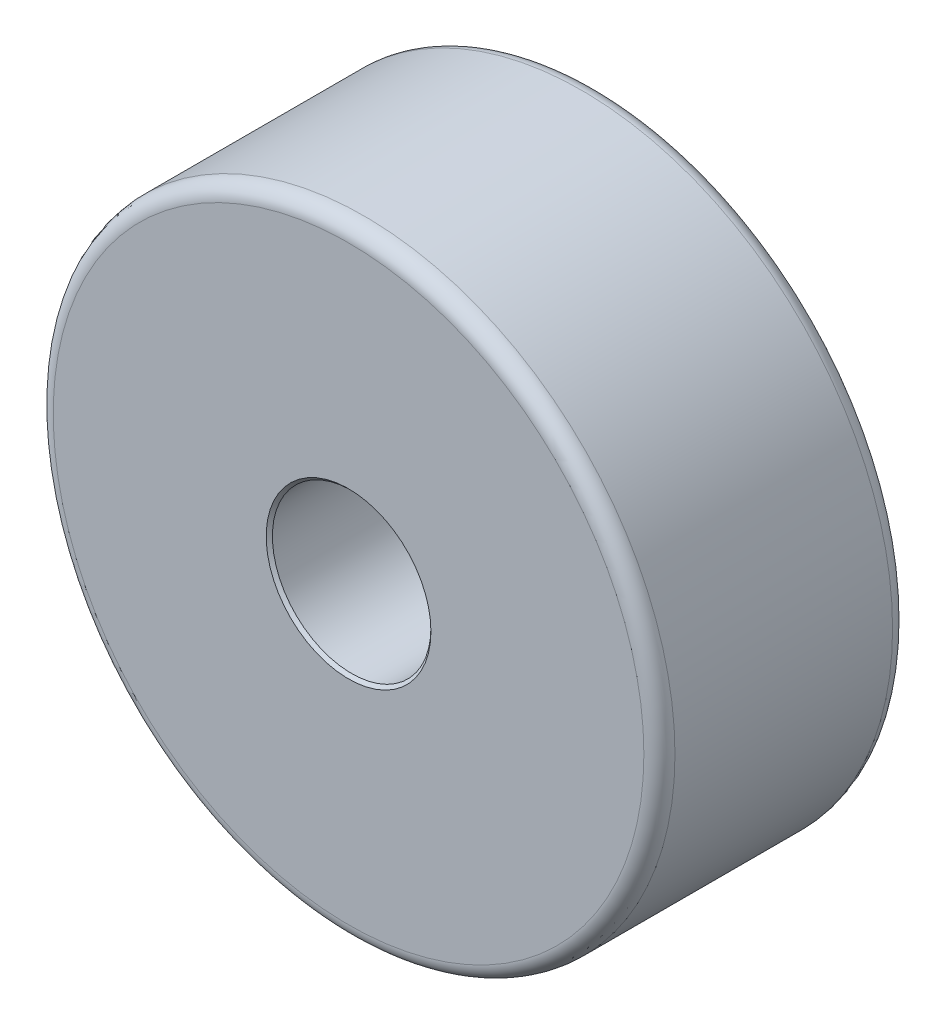
from build123d import *

# Parameters (mm, degrees)
SKETCH1_R           = 100
SKETCH1_R_2         = 25.5
BOSS_EXTRUDE1_DEPTH = 80
FILLET1_R           = 5
CHAMFER1_SIZE       = 1


with BuildPart() as part:
    # Sketch1 → Boss-Extrude1 (new body)
    with BuildSketch(Plane.XY):
        Circle(SKETCH1_R)
        Circle(SKETCH1_R_2, mode=Mode.SUBTRACT)
    extrude(amount=BOSS_EXTRUDE1_DEPTH)

    # Fillet1
    fillet1_edges = [part.edges().sort_by_distance(p)[0] for p in [
        (-100, 0, 0),
        (-100, 0, 80),
    ]]
    fillet(fillet1_edges, radius=FILLET1_R)

    # Chamfer1
    chamfer1_edges = [part.edges().sort_by_distance(p)[0] for p in [
        (-25.5, 0, 0),
        (-25.5, 0, 80),
    ]]
    chamfer(chamfer1_edges, length=CHAMFER1_SIZE)


solid = part.part
